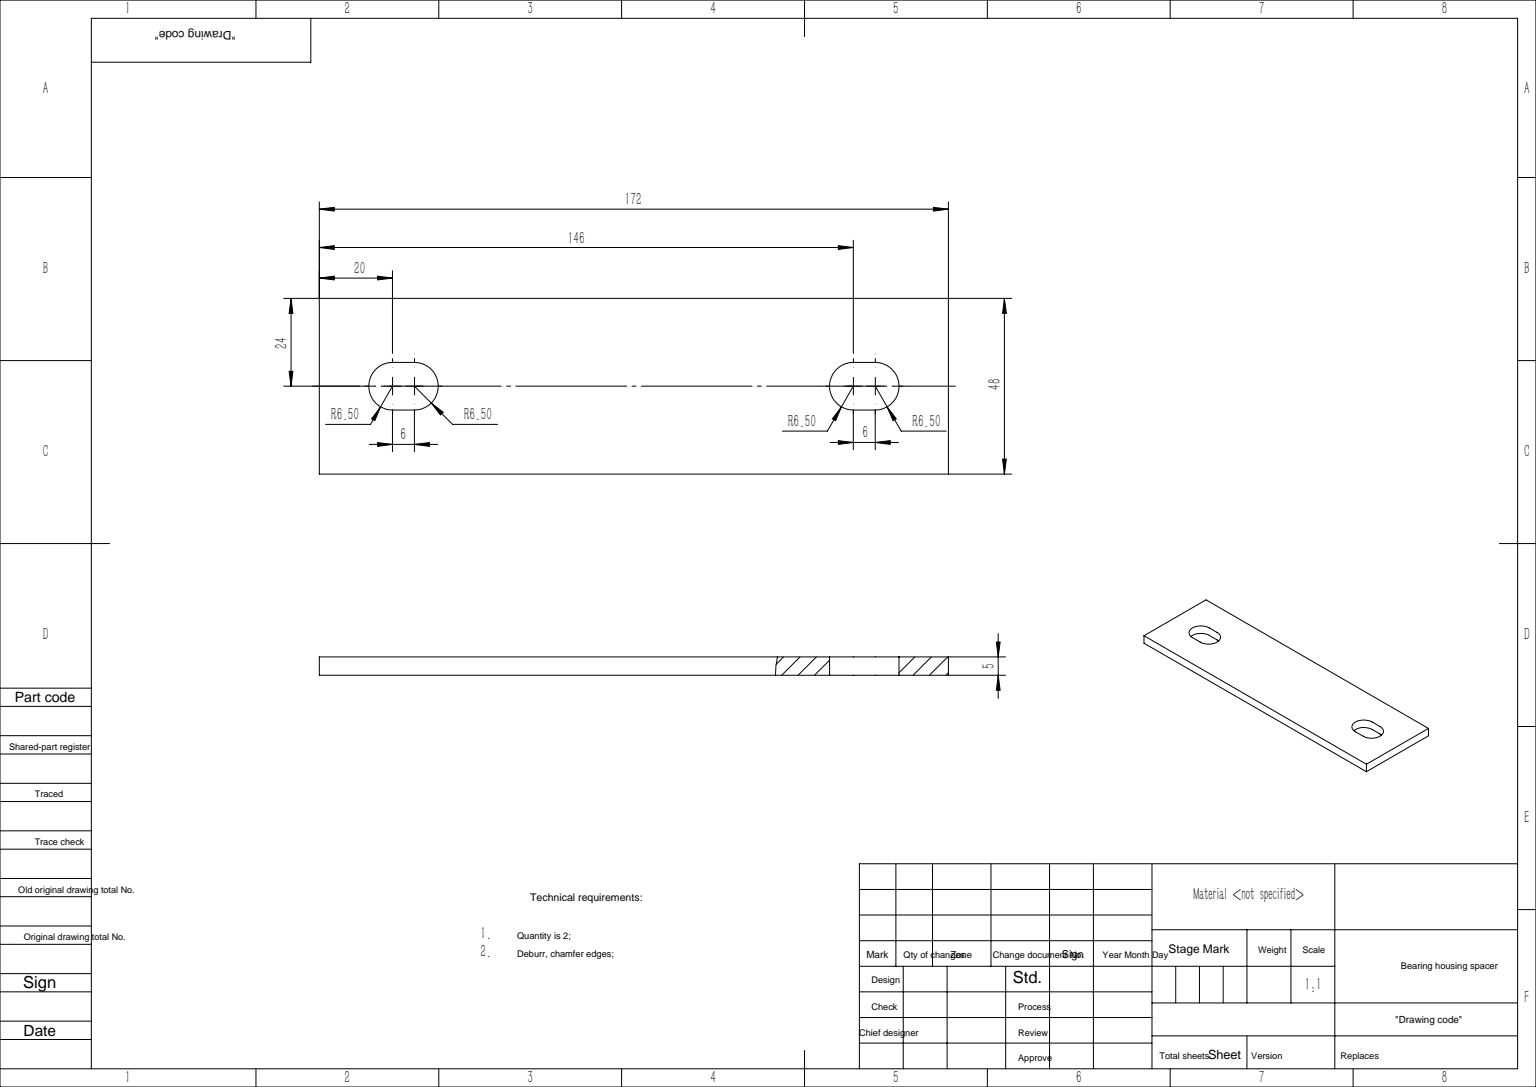
from build123d import *

# Parameters (mm, degrees)
SKETCH_1_W          = 172
SKETCH_1_H          = 48
EXTRUDE_1_DEPTH     = 5
CUT_EXTRUDE_1_DEPTH = 90.425947018


with BuildPart() as part:
    # 草图1 → 凸台-拉伸1 (new body)
    with BuildSketch(Plane(origin=(0, 0, 0), x_dir=(1, 0, 0), z_dir=(0, 1, 0))):
        Rectangle(SKETCH_1_W, SKETCH_1_H)
    extrude(amount=EXTRUDE_1_DEPTH)

    # 草图2 → 切除-拉伸1 (cut, through all)
    with BuildSketch(Plane(origin=(0, 5, 0), x_dir=(1, 0, 0), z_dir=(0, 1, 0))):
        with BuildLine():
            Line((66, -6.5), (60, -6.5))
            ThreePointArc((60, -6.5), (53.5, 0), (60, 6.5))
            Line((60, 6.5), (66, 6.5))
            ThreePointArc((66, 6.5), (72.5, 0), (66, -6.5))
        make_face()
        with BuildLine():
            Line((-66, 6.5), (-60, 6.5))
            ThreePointArc((-60, 6.5), (-53.5, 0), (-60, -6.5))
            Line((-60, -6.5), (-66, -6.5))
            ThreePointArc((-66, -6.5), (-72.5, 0), (-66, 6.5))
        make_face()
    extrude(amount=-CUT_EXTRUDE_1_DEPTH, mode=Mode.SUBTRACT)


solid = part.part
